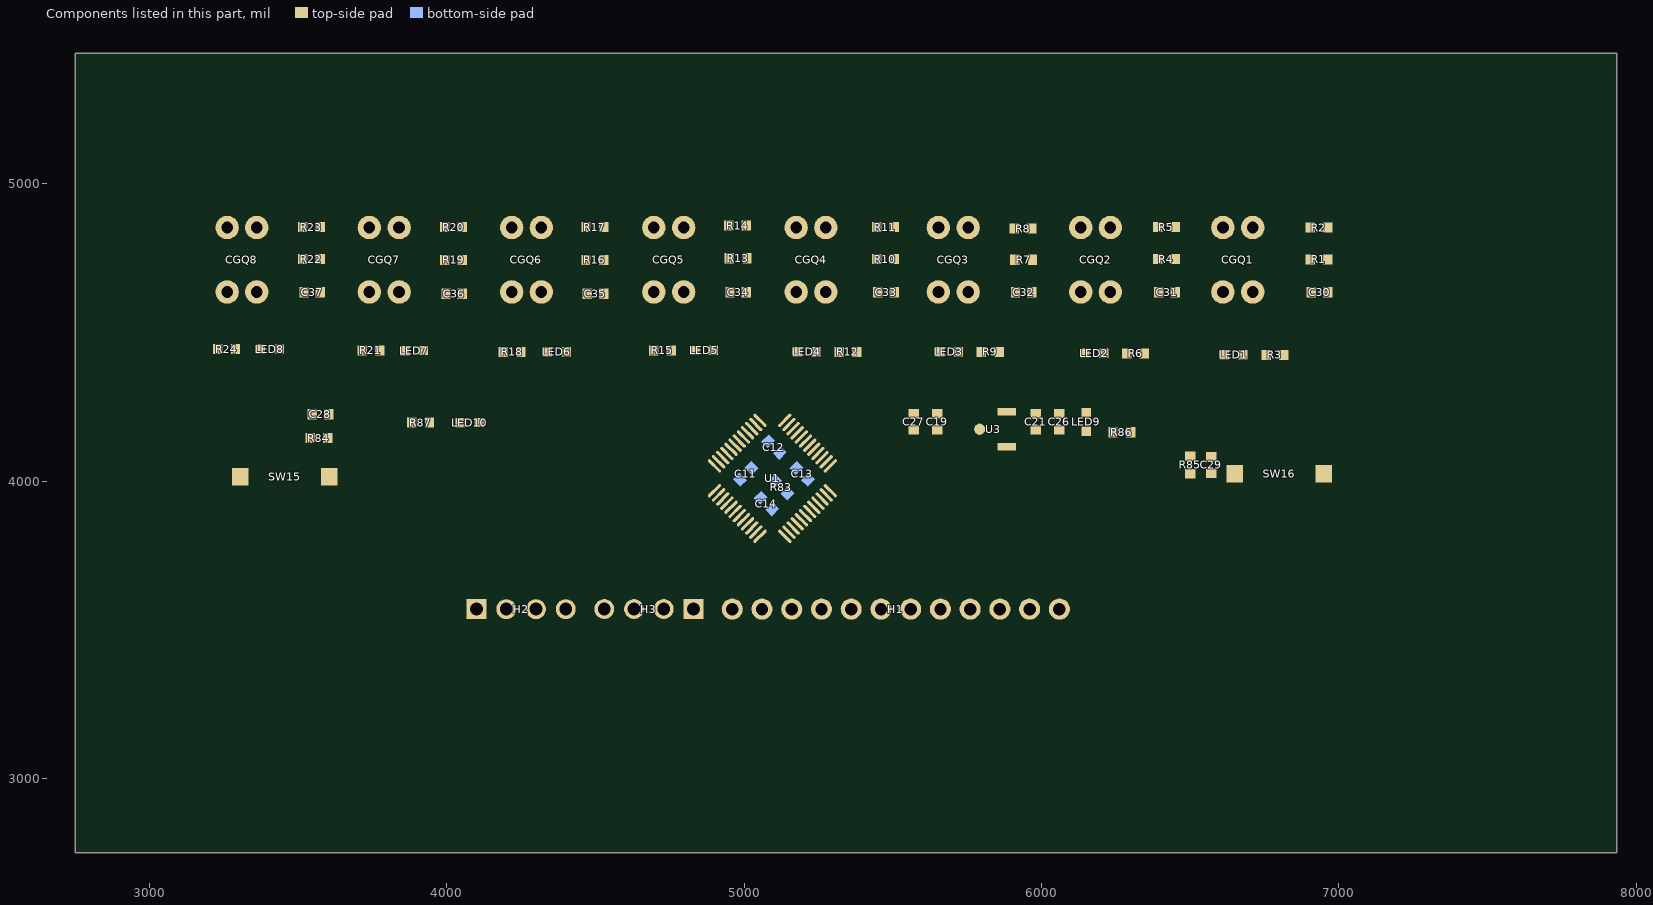
[diagram p0: the components of this part, seen from the top]
# Altium PCB MISC51279.pcbdoc (part 3 of 3)
Units mil, origin at the board's own origin, x right, y up, seen from the top; angles counter-clockwise.
Board outline 5185 x 2690 mil, 2 copper layers (Top Layer, Bottom Layer), stack 62.206 mil thick; 72 components, 47 nets, 221 pads, 129 vias.

## Other copper (continued)
Bottom Layer:
  region net OUT1: 6055,3618.24 6065,3618.24 6065.12,3615.41 6065.48,3612.99 6066.07,3610.94 6066.85,3609.2 6067.83,3607.72 6068.98,3606.45 6070.29,3605.33 6071.74,3604.31 6078.65,3600.18 6080.58,3598.87 6082.55,3597.35 6084.55,3595.55 6086.57,3593.44 6033.43,3593.44 6035.45,3595.55 6037.45,3597.35 6039.42,3598.87 6041.35,3600.18 6048.26,3604.31 6049.71,3605.33 6051.02,3606.45 6052.17,3607.72 6053.15,3609.2 6053.93,3610.94 6054.52,3612.99 6054.88,3615.41
  region net OUT2: 5955,3618.24 5965,3618.24 5965.12,3615.41 5965.48,3612.99 5966.07,3610.94 5966.85,3609.2 5967.83,3607.72 5968.98,3606.45 5970.29,3605.33 5971.74,3604.31 5978.65,3600.18 5980.58,3598.87 5982.55,3597.35 5984.55,3595.55 5986.57,3593.44 5933.43,3593.44 5935.45,3595.55 5937.45,3597.35 5939.42,3598.87 5941.35,3600.18 5948.26,3604.31 5949.71,3605.33 5951.02,3606.45 5952.17,3607.72 5953.15,3609.2 5953.93,3610.94 5954.52,3612.99 5954.88,3615.41
  region net OUT3: 5855,3618.24 5865,3618.24 5865.12,3615.41 5865.48,3612.99 5866.07,3610.94 5866.85,3609.2 5867.83,3607.72 5868.98,3606.45 5870.29,3605.33 5871.74,3604.31 5878.65,3600.18 5880.58,3598.87 5882.55,3597.35 5884.55,3595.55 5886.57,3593.44 5833.43,3593.44 5835.45,3595.55 5837.45,3597.35 5839.42,3598.87 5841.35,3600.18 5848.26,3604.31 5849.71,3605.33 5851.02,3606.45 5852.17,3607.72 5853.15,3609.2 5853.93,3610.94 5854.52,3612.99 5854.88,3615.41
  region net OUT4: 5755,3618.24 5765,3618.24 5765.12,3615.41 5765.48,3612.99 5766.07,3610.94 5766.85,3609.2 5767.83,3607.72 5768.98,3606.45 5770.29,3605.33 5771.74,3604.31 5778.65,3600.18 5780.58,3598.87 5782.55,3597.35 5784.55,3595.55 5786.57,3593.44 5733.43,3593.44 5735.45,3595.55 5737.45,3597.35 5739.42,3598.87 5741.35,3600.18 5748.26,3604.31 5749.71,3605.33 5751.02,3606.45 5752.17,3607.72 5753.15,3609.2 5753.93,3610.94 5754.52,3612.99 5754.88,3615.41
  region net OUT5: 5655,3618.24 5665,3618.24 5665.12,3615.41 5665.48,3612.99 5666.07,3610.94 5666.85,3609.2 5667.83,3607.72 5668.98,3606.45 5670.29,3605.33 5671.74,3604.31 5678.65,3600.18 5680.58,3598.87 5682.55,3597.35 5684.55,3595.55 5686.57,3593.44 5633.43,3593.44 5635.45,3595.55 5637.45,3597.35 5639.42,3598.87 5641.35,3600.18 5648.26,3604.31 5649.71,3605.33 5651.02,3606.45 5652.17,3607.72 5653.15,3609.2 5653.93,3610.94 5654.52,3612.99 5654.88,3615.41
  region net OUT6: 5555,3618.24 5565,3618.24 5565.12,3615.41 5565.48,3612.99 5566.07,3610.94 5566.85,3609.2 5567.83,3607.72 5568.98,3606.45 5570.29,3605.33 5571.74,3604.31 5578.65,3600.18 5580.58,3598.87 5582.55,3597.35 5584.55,3595.55 5586.57,3593.44 5533.43,3593.44 5535.45,3595.55 5537.45,3597.35 5539.42,3598.87 5541.35,3600.18 5548.26,3604.31 5549.71,3605.33 5551.02,3606.45 5552.17,3607.72 5553.15,3609.2 5553.93,3610.94 5554.52,3612.99 5554.88,3615.41
  region net OUT7: 5455,3618.24 5465,3618.24 5465.12,3615.41 5465.48,3612.99 5466.07,3610.94 5466.85,3609.2 5467.83,3607.72 5468.98,3606.45 5470.29,3605.33 5471.74,3604.31 5478.65,3600.18 5480.58,3598.87 5482.55,3597.35 5484.55,3595.55 5486.57,3593.44 5433.43,3593.44 5435.45,3595.55 5437.45,3597.35 5439.42,3598.87 5441.35,3600.18 5448.26,3604.31 5449.71,3605.33 5451.02,3606.45 5452.17,3607.72 5453.15,3609.2 5453.93,3610.94 5454.52,3612.99 5454.88,3615.41
  region net OUT8: 5355,3618.24 5365,3618.24 5365.12,3615.41 5365.48,3612.99 5366.07,3610.94 5366.85,3609.2 5367.83,3607.72 5368.98,3606.45 5370.29,3605.33 5371.74,3604.31 5378.65,3600.18 5380.58,3598.87 5382.55,3597.35 5384.55,3595.55 5386.57,3593.44 5333.43,3593.44 5335.45,3595.55 5337.45,3597.35 5339.42,3598.87 5341.35,3600.18 5348.26,3604.31 5349.71,3605.33 5351.02,3606.45 5352.17,3607.72 5353.15,3609.2 5353.93,3610.94 5354.52,3612.99 5354.88,3615.41
  region net 3V3: 4964.49,3967.51 4947.51,3984.49 4951.99,3989.47 4955.9,3994.92 4959.2,4000.75 4961.85,4006.9 4986.9,3981.85 4980.75,3979.2 4974.92,3975.9 4969.47,3971.99 4964.49,3967.51
  region net 3V3: 4965.48,4018.47 4972.55,4025.54 4974.42,4024.82 4976.41,4024.59 4978.39,4024.88 4980.24,4025.66 4981.82,4026.88 4964.15,4009.2 4965.37,4010.79 4966.15,4012.63 4966.43,4014.61 4966.21,4016.61 4965.48,4018.47
  region net GND: 4990.29,4064.55 5004.43,4078.69 5008.51,4075.13 5013.04,4072.15 5017.93,4069.81 5023.1,4068.15 5000.82,4045.88 4999.17,4051.04 4996.83,4055.93 4993.85,4060.46 4990.29,4064.55
  region net 3V3: 5114.49,4120.28 5124.49,4123.07 5125.43,4118.91 5127.02,4114.96 5129.23,4111.31 5131.99,4108.07 5106.99,4105.28 5109.75,4108.53 5111.95,4112.17 5113.55,4116.13 5114.49,4120.28
  region net 3V3: 5156.88,4107.51 5154.1,4083.51 5147.7,4083.18 5141.37,4082.18 5135.17,4080.52 5129.19,4078.23 5123.48,4075.33 5118.1,4071.85 5120.88,4119.18 5126.26,4115.69 5131.97,4112.79 5137.96,4110.5 5144.15,4108.85 5150.48,4107.85 5156.88,4107.51
  region net GND: 5053.84,4093.68 5039.7,4107.82 5044.87,4113.5 5049.47,4119.64 5053.48,4126.19 5056.85,4133.1 5079.12,4110.82 5072.22,4107.46 5065.67,4103.45 5059.52,4098.84 5053.84,4093.68
  region net 3V3: 5226.49,3970.9 5202.49,3968.12 5202.15,3974.52 5201.15,3980.85 5199.5,3987.04 5197.21,3993.03 5194.31,3998.74 5190.82,4004.12 5238.15,4006.9 5234.67,4001.52 5231.77,3995.81 5229.48,3989.83 5227.82,3983.63 5226.82,3977.3 5226.49,3970.9
  region net 3V3: 5241.51,4049.51 5258.49,4032.54 5252.86,4026.58 5247.58,4020.31 5242.67,4013.74 5238.15,4006.9 5215.88,4029.18 5222.72,4033.7 5229.28,4038.61 5235.55,4043.88 5241.51,4049.51
  region net 3V3: 5244.44,4008.12 5236.86,3998.12 5232.71,3997.18 5228.76,3995.58 5225.11,3993.38 5221.86,3990.62 5229.44,4015.62 5232.68,4012.86 5236.33,4010.65 5240.28,4009.06 5244.44,4008.12
  region net GND: 5158.33,3994.19 5144.19,4008.33 5147.46,4012.07 5150.21,4016.2 5152.38,4020.66 5153.95,4025.37 5154.89,4030.24 5155.17,4035.2 5154.79,4040.15 5174.12,4020.82 5169.92,4016.19 5166.21,4011.15 5163.02,4005.77 5160.39,4000.1 5158.33,3994.19
  region net 3V3: 5131.88,3912 5129.1,3888 5119.93,3887.61 5110.84,3886.45 5101.87,3884.53 5093.1,3881.85 5095.88,3929.18 5100.93,3924.66 5106.47,3920.75 5112.4,3917.5 5118.67,3914.93 5125.19,3913.09 5131.88,3912
  region net 3V3: 5107,3870.9 5083,3868.12 5082.65,3874.55 5081.6,3880.91 5079.87,3887.12 5077.48,3893.11 5074.45,3898.79 5070.82,3904.12 5118.15,3906.9 5114.82,3901.47 5112.04,3895.73 5109.85,3889.75 5108.27,3883.57 5107.32,3877.27 5107,3870.9
  region net 3V3: 5057.1,3888 5059.88,3912 5066.57,3913.09 5073.09,3914.93 5079.35,3917.5 5085.29,3920.75 5090.83,3924.66 5095.88,3929.18 5093.1,3881.85 5084.32,3884.53 5075.36,3886.45 5066.26,3887.61 5057.1,3888
  region net GND: 5001.85,3945 5026.9,3965 5036.97,3965.35 5046.99,3966.4 5056.9,3968.15 5031.85,3943.1 5021.88,3944.15 5011.87,3944.79 5001.85,3945
  region net $1N3211: 5163.54,3948.54 5156.46,3941.46 5154.27,3941.61 5152.1,3941.22 5150.09,3940.32 5148.36,3938.96 5166.04,3956.64 5164.68,3954.91 5163.78,3952.9 5163.39,3950.73 5163.54,3948.54
  region net GND: 5077.93,4012.93 5092.07,4027.07 5094.23,4025.36 5096.71,4024.17 5099.4,4023.57 5102.15,4023.59 5104.83,4024.22 5080.78,4000.17 5081.41,4002.85 5081.43,4005.6 5080.83,4008.29 5079.64,4010.77 5077.93,4012.93
  region net 3V3: 5083,3874.41 5107,3874.41 5107.01,3860 5082.99,3860
  region net 3V3: 5243.65,3998.12 5243.65,4008.12 5244.79,4008.21 5245.92,4008.46 5248.14,4009.37 5250.21,4010.65 5252.06,4012.12 5252.06,3994.11 5250.21,3995.58 5248.14,3996.86 5245.92,3997.77 5244.79,3998.03
  region net 3V3: 5124.49,4115 5114.49,4124.12 5114.24,4128.34 5113.66,4132.53 5128.53,4123.41 5127.35,4122.92 5126.41,4122.21 5125.7,4121.29 5125.19,4120.22 5124.84,4119.02 5124.62,4117.72
  region net 3V3: 4966.35,4027.01 4966.35,4017.01 4965.21,4016.92 4964.08,4016.66 4961.86,4015.76 4959.79,4014.47 4957.94,4013 4957.94,4031.01 4959.79,4029.54 4961.86,4028.26 4964.08,4027.35 4965.21,4027.1
  region net $1N3211: 5163.65,3940 5163.65,3950 5164.79,3950.09 5165.92,3950.34 5168.14,3951.25 5170.21,3952.53 5172.06,3954.01 5172.06,3935.99 5170.21,3937.47 5168.14,3938.75 5165.92,3939.66 5164.79,3939.91
  region net OUT8: 3440,4373.65 3430,4373.65 3429.91,4374.79 3429.66,4375.92 3428.75,4378.14 3427.47,4380.21 3425.99,4382.06 3444.01,4382.06 3442.53,4380.21 3441.25,4378.14 3440.34,4375.92 3440.09,4374.79
  region net OUT7: 3924.98,4366.09 3914.98,4366.09 3914.89,4367.23 3914.63,4368.36 3913.73,4370.58 3912.44,4372.65 3910.97,4374.49 3928.98,4374.49 3927.51,4372.65 3926.23,4370.58 3925.32,4368.36 3925.07,4367.23
  region net OUT6: 4407.73,4364.05 4397.73,4364.05 4397.64,4365.19 4397.38,4366.32 4396.47,4368.54 4395.19,4370.61 4393.72,4372.46 4411.73,4372.46 4410.26,4370.61 4408.98,4368.54 4408.07,4366.32 4407.82,4365.19
  region net OUT5: 4900.17,4369.07 4890.17,4369.07 4890.08,4370.21 4889.82,4371.35 4888.91,4373.56 4887.63,4375.63 4886.16,4377.48 4904.17,4377.48 4902.7,4375.63 4901.42,4373.56 4900.51,4371.35 4900.26,4370.21
  region net OUT3: 5661.02,4364.01 5651.02,4364.01 5650.93,4365.15 5650.68,4366.28 5649.77,4368.5 5648.49,4370.57 5647.02,4372.42 5665.03,4372.42 5663.56,4370.57 5662.27,4368.5 5661.37,4366.28 5661.11,4365.15
  region net OUT2: 6149.75,4359.01 6139.75,4359.01 6139.66,4360.15 6139.41,4361.28 6138.5,4363.5 6137.22,4365.57 6135.75,4367.42 6153.76,4367.42 6152.29,4365.57 6151,4363.5 6150.1,4361.28 6149.84,4360.15
  region net OUT1: 6618.5,4354.02 6608.5,4354.02 6608.41,4355.15 6608.16,4356.29 6607.25,4358.5 6605.97,4360.57 6604.5,4362.42 6622.51,4362.42 6621.04,4360.57 6619.76,4358.5 6618.85,4356.29 6618.59,4355.15
  region net 3V3: 5262,4185.59 5238,4185.59 5237.99,4200 5262.01,4200
  region net 3V3: 5492.28,4184.43 5492.28,4160.43 5477.87,4160.42 5477.87,4184.44
  region net 3V3: 6486.96,4160.43 6482.02,4184.43 6482.67,4184.32 6483.29,4184.01 6484.5,4182.92 6485.65,4181.43 6486.74,4179.81 6487.76,4178.31 6488.72,4177.21 6489.17,4176.89 6489.61,4176.77 6490.03,4176.88 6490.43,4177.25 6495.36,4158.92 6493.45,4159.55 6491.23,4160.03 6488.97,4160.33
  region net 3V3: 4956.7,3833.67 4973.67,3816.7 4963.49,3806.51 4946.51,3823.49
  region net GND: 5153.12,4017.26 5167.26,4003.12 5165.45,4001.19 5163.84,3999.25 5161.23,3995.67 5159.44,3992.9 5158.49,3991.51 5141.51,4008.49 5142.9,4009.44 5145.67,4011.23 5149.25,4013.84 5151.19,4015.45
  region net GND: 5011.7,4071.41 5000.37,4054.47 4999.45,4055.52 4998.72,4056.57 4997.5,4058.45 4996.86,4059.17 4996.08,4059.67 4995.1,4059.91 4993.83,4059.82 5003.2,4074.79 5003.74,4073.73 5004.57,4073.13 5005.63,4072.85 5006.84,4072.75 5009.41,4072.54 5010.63,4072.16
  region net GND: 5014.41,3965 5014.41,3945 5011.76,3944.91 5009.26,3944.69 5004.88,3944 5001.66,3943.31 5000,3942.99 5000,3967.01 5001.66,3966.69 5004.88,3966 5009.26,3965.31 5011.76,3965.09
  region net GND: 5095,4040.59 5075,4040.59 5074.91,4043.24 5074.69,4045.74 5074,4050.12 5073.31,4053.34 5072.99,4055 5097.01,4055 5096.69,4053.34 5096,4050.12 5095.31,4045.74 5095.09,4043.24
  region net GND: 5047.57,4115.69 5055.09,4094.92 5054.4,4094.35 5053.72,4093.97 5052.37,4093.71 5051.03,4093.9 5049.72,4094.29 5048.45,4094.66 5047.21,4094.76 5046.62,4094.64 5046.03,4094.36 5045.46,4093.89 5044.91,4093.21 5040.94,4110.43 5042.13,4109.96 5043.07,4110 5043.84,4110.45 5044.51,4111.23 5045.82,4113.37 5046.61,4114.56
  region net OUT4: 5193.75,4371.98 5186.67,4364.9 5185.81,4365.65 5184.82,4366.27 5182.62,4367.19 5180.24,4367.75 5177.9,4368.02 5190.63,4380.75 5190.9,4378.41 5191.46,4376.03 5192.38,4373.83 5193,4372.84
  region net 3V3: 5166,4083.51 5175.64,4083.12 5185.22,4081.96 5194.68,4080.04 5203.95,4077.35 5212.97,4073.94 5221.69,4069.81 5230.05,4064.99 5238,4059.51 5250,4093.55 5238,4131.51 5230.05,4126.04 5221.69,4121.22 5212.97,4117.09 5203.95,4113.67 5194.68,4110.99 5185.22,4109.06 5175.64,4107.9 5166,4107.51 5166,4083.51
  region net 3V3: 5056.97,3912 5045.04,3912.33 5033.15,3913.3 5021.32,3914.92 5009.61,3917.18 4998.03,3920.08 4986.63,3923.6 4975.44,3927.74 4964.49,3932.49 4947.51,3915.51 4952.23,3906.82 4956.36,3897.82 4959.88,3888.58 4962.79,3879.12 4965.06,3869.49 4966.69,3859.73 4967.67,3849.89 4968,3840 4992,3840 4995.28,3846.9 4999.22,3853.45 5003.78,3859.58 5008.92,3865.23 5014.59,3870.36 5020.73,3874.9 5027.29,3878.82 5034.2,3882.08 5041.4,3884.65 5048.81,3886.51 5056.37,3887.63 5064,3888 5056.97,3912

## Silkscreen, mask and mechanical layers (free items; w line width, h text height)
Top Silkscreen Layer:
  lines w10: 4041.73,3620 4041.73,3725 6119.99,3725 6119.99,3619.99 ; 4150.93,3620 4150.93,3725 ; 4250,3620 4250,3725 ; 4350,3625 4350,3725 ; 4458.27,3620 4458.27,3725 ; 4471.42,3620.18 4471.42,3725 ; 4579.83,3620.18 4579.83,3725 ; 4679.69,3620.18 4679.69,3724.69 4680,3725 ; 4778.76,3620.18 4778.76,3725 ; 4885,3725 4887.96,3722.04 4887.96,3620.18 ; 4900.16,3619.21 4900.16,3725 ; 5010,3725 5010.62,3724.38 5010.62,3619.21 ; 5107.71,3619.21 5107.71,3725 ; 5210,3625 5210,3725 ; 5310.16,3619.21 5310.16,3725 ; 5410,3725 5410.62,3724.38 5410.62,3619.21 ; 5507.71,3619.21 5507.71,3725 ; 5610,3625 5610,3725 ; 5705.16,3619.21 5705.16,3725 ; 5810,3725 5810.62,3724.38 5810.62,3619.21 ; 5907.71,3619.21 5907.71,3725 ; 6010,3625 6010,3725
  text "RESET" at 6726.85,4157.5 h45
  text "PB1" at 4035.05,4112.5 h45
  text "PB0" at 3172.99,3992.5 h45
  text "GND" at 4165,3655 h35
  text "GND" at 4694.69,3655.18 h35
  text "SWC" at 5025,3655 h35
  text "GND" at 5125,3655 h35
  text "VCC" at 5220,3655 h35
  text "OUT8" at 5315,3655 h35
  text "OUT7" at 5420,3655 h35
  text "OUT6" at 5515,3655 h35
  text "OUT5" at 5615,3655 h35
  text "OUT4" at 5715,3655 h35
  text "OUT3" at 5815,3655 h35
  text "OUT2" at 5915,3655 h35
  text "OUT1" at 6025,3655 h35
  text "3V3" at 4050,3650 h45
  text "SCL" at 4260,3650 h45
  text "SDA" at 4365,3650 h45
  text "RX" at 4505,3650 h45
  text "TX" at 4600,3650 h45
  text "SWD" at 4910,3650 h45
  text "3V3" at 4790,3645 h45
Mechanical Layer:
  lines w0.1: 3789.29,3995.04 cw(c3850.31,3995.04) 3850.31,4056.06 4712.52,4056.06 cw(c4712.52,3995.04) 4773.54,3995.04 cw(c4712.52,3995.04) 4712.52,3934.02 3850.31,3934.02 cw(c3850.31,3995.04) 3789.29,3995.04 ; 5403.46,3995.04 cw(c5464.49,3995.04) 5464.49,4056.06 6326.69,4056.06 cw(c6326.69,3995.04) 6387.72,3995.04 cw(c6326.69,3995.04) 6326.69,3934.02 5464.49,3934.02 cw(c5464.49,3995.04) 5403.46,3995.04